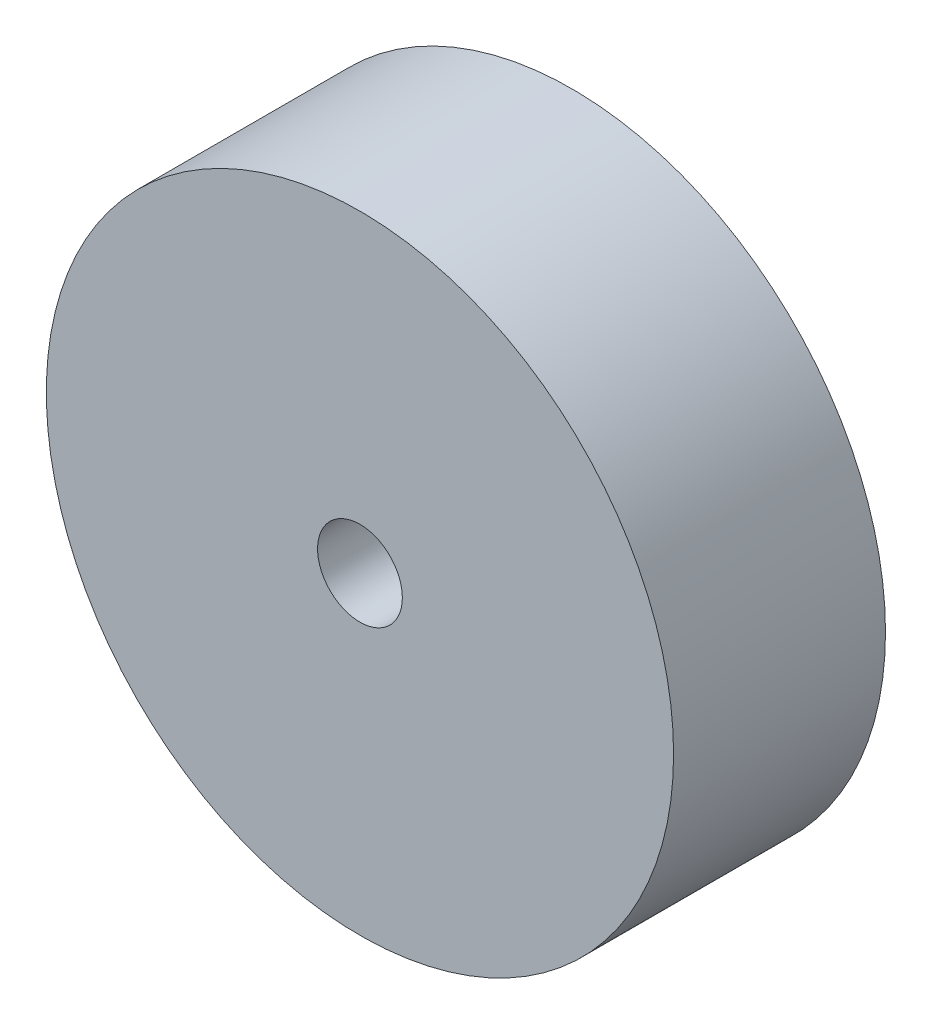
from build123d import *

# Parameters (mm, degrees)
SKETCH1_R           = 7.4
SKETCH1_R_2         = 1
BOSS_EXTRUDE1_DEPTH = 5


with BuildPart() as part:
    # Sketch1 → Boss-Extrude1 (new body)
    with BuildSketch(Plane.XY):
        Circle(SKETCH1_R)
        Circle(SKETCH1_R_2, mode=Mode.SUBTRACT)
    extrude(amount=BOSS_EXTRUDE1_DEPTH)


solid = part.part
